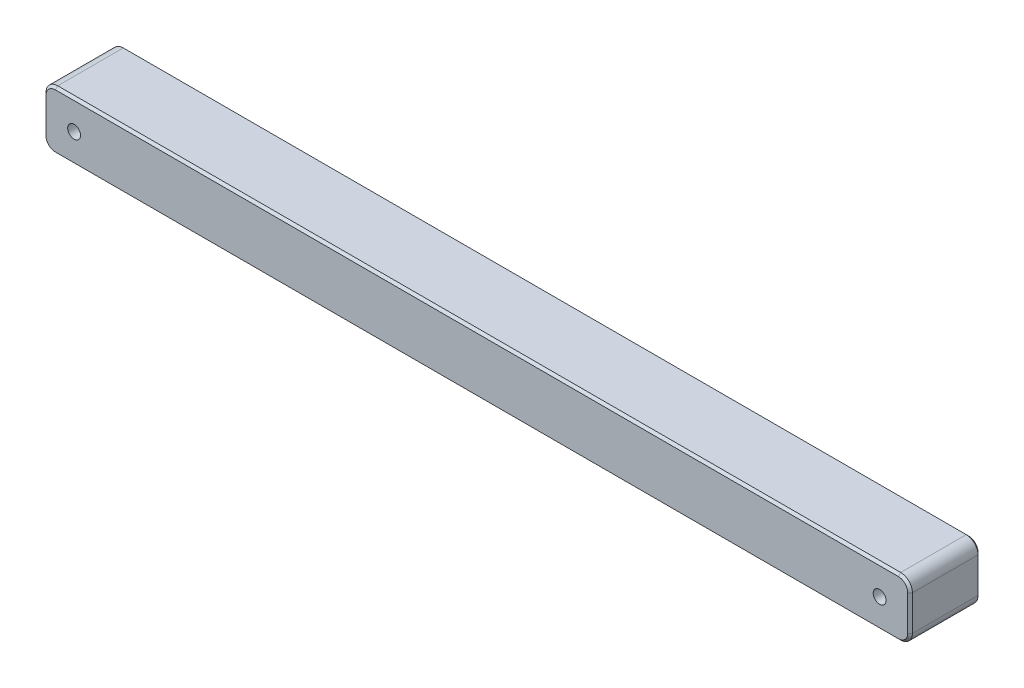
SolidWorks part; units mm, degrees
ref_plane "Front Plane" through (0, 0, 0) normal (0, 0, 1) x (1, 0, 0)
ref_plane "Top Plane" through (0, 0, 0) normal (0, 1, 0) x (1, 0, 0)
ref_plane "Right Plane" through (0, 0, 0) normal (1, 0, 0) x (0, 0, -1)
sketch "Sketch1" plane through (0, 0, 0) normal (0, 0, 1) x (1, 0, 0)
  line L1 (-185, 12.5) -> (185, 12.5)
  line L2 (-185, 12.5) -> (-185, -12.5)
  line L3 (-185, -12.5) -> (185, -12.5)
  line L4 (185, 12.5) -> (185, -12.5)
  line L5 (-185, 12.5) -> (185, -12.5) construction
  line L6 (-185, -12.5) -> (185, 12.5) construction
  point P0 (0, 0)
  dimension "D1" = 370
  dimension "D2" = 25
extrude "Boss-Extrude1" add sketch "Sketch1" along normal mid plane 30
fillet "Fillet1" radius 5 4 edges at (-185, 12.5, 0) (-185, -12.5, 0) (185, -12.5, 0) (185, 12.5, 0)
chamfer "Chamfer1" distance 1 angle 45 16 edges at (183.5355, 11.0355, 15) (185, 0, 15) (183.5355, -11.0355, 15) (0, -12.5, 15) (-183.5355, -11.0355, 15) (-185, 0, 15) (-183.5355, 11.0355, 15) (0, 12.5, 15) (0, 12.5, -15) (-183.5355, 11.0355, -15) (183.5355, 11.0355, -15) (-185, 0, -15) (185, 0, -15) (-183.5355, -11.0355, -15) (183.5355, -11.0355, -15) (0, -12.5, -15)
hole_wizard "Hole size per socket head cap screw type 1" positions "Sketch3" profile "Sketch2" counterbore size "M5" standard "Gb" end condition through all
sketch "Sketch3" plane through (0, 0, -15) normal (0, 0, -1) x (-1, 0, 0)
  line L0 (0, 0) -> (0, 75.1992) construction
  line L2 (0, 0) -> (-227.5853, 0) construction
  point P0 (-172, 0)
  point P11 (172, 0)
  dimension "D1" = 172
sketch "Sketch2" plane through (172, 0, -15) normal (1, 0, 0) x (0, 1, 0)
  line L0 (0, 0) -> (0, 30)
  line L1 (0, 30) -> (2.75, 30)
  line L3 (2.75, 30) -> (2.75, 5.7)
  line L4 (2.75, 5.7) -> (5, 5.7)
  line L5 (5, 5.7) -> (5, 0)
  line L7 (5, 0) -> (0, 0)
  line L11 (0, -6.35) -> (0, 107.95) construction
  dimension "通孔孔直径" = 5.5
  dimension "通孔孔深度" = 30
  dimension "柱形沉头孔直径" = 10
  dimension "柱形沉头孔深度" = 5.7
